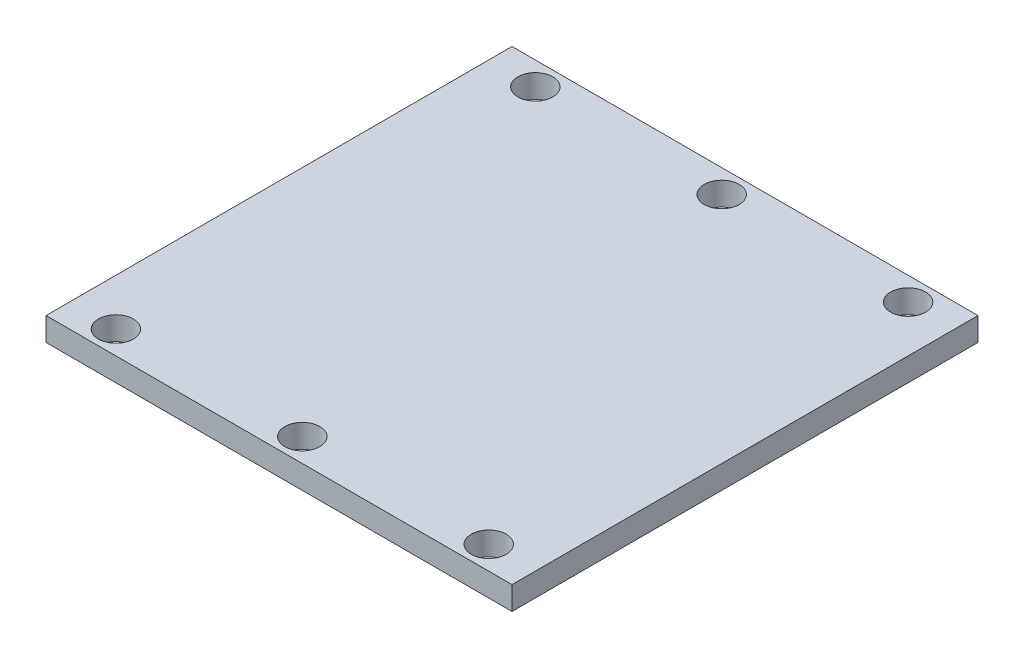
SolidWorks part; units mm, degrees
ref_plane "Front Plane" through (0, 0, 0) normal (0, 0, 1) x (1, 0, 0)
ref_plane "Top Plane" through (0, 0, 0) normal (0, 1, 0) x (1, 0, 0)
ref_plane "Right Plane" through (0, 0, 0) normal (1, 0, 0) x (0, 0, -1)
sketch "Sketch1" plane through (0, 0, 0) normal (0, 1, 0) x (1, 0, 0)
  line L1 (-100, 100) -> (100, 100)
  line L2 (-100, 100) -> (-100, -100)
  line L3 (-100, -100) -> (100, -100)
  line L4 (100, 100) -> (100, -100)
  line L5 (-100, 100) -> (100, -100) construction
  line L6 (-100, -100) -> (100, 100) construction
  point P0 (0, 0)
  dimension "D1" = 200
  dimension "D2" = 200
extrude "Boss-Extrude1" add sketch "Sketch1" along normal mid plane 10
sketch "Sketch2" plane through (0, 5, 0) normal (0, 1, 0) x (1, 0, 0)
  line L0 (0, 90) -> (0, -90) construction
  line L1 (80, 90) -> (-80, 90) construction
  line L2 (80, 90) -> (80, -90) construction
  line L3 (80, -90) -> (-80, -90) construction
  line L4 (-80, 90) -> (-80, -90) construction
  line L5 (80, 90) -> (-80, -90) construction
  line L6 (80, -90) -> (-80, 90) construction
  circle A0 centre (80, 90) radius 7.5
  point P0 (0, 0)
  dimension "D3" = 15
  dimension "D1" = 180
  dimension "D2" = 160
extrude "Cut-Extrude1" cut sketch "Sketch2" against normal blind 10
pattern_linear "LPattern1" count 2 spacing 180 along (0, 0, 1) count 3 spacing 80 along (-1, 0, 0) of "Cut-Extrude1"
